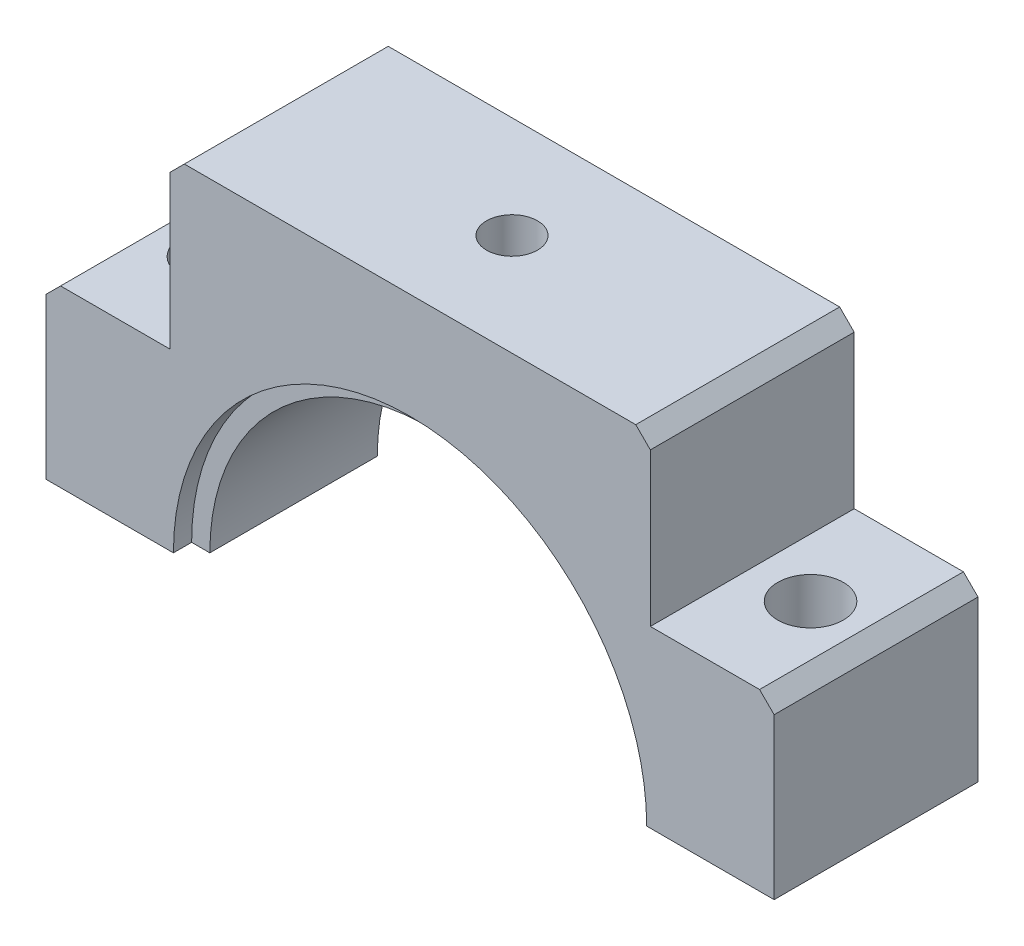
from build123d import *

# Parameters (mm, degrees)
BOSS_EXTRUDE1_DEPTH       = 28
CHAMFER1_SIZE             = 2
M8X1_0_TAPPED_HOLE1_D     = 7
M8X1_0_TAPPED_HOLE1_DEPTH = 13
M8X1_0_TAPPED_HOLE1_TIP   = 2.103012167
HOLE2_D                   = 9
SKETCH15_R                = 32.5
CUT_EXTRUDE3_DEPTH        = 2.5
CUT_EXTRUDE4_START        = -2.5
SKETCH16_R                = 32.5
CUT_EXTRUDE4_DEPTH        = 2.5
HOLE3_D                   = 4


with BuildPart() as part:
    # Sketch1 → Boss-Extrude1 (new body)
    with BuildSketch(Plane.XY):
        with BuildLine():
            Line((-50, 24), (-33, 24))
            Line((-33, 24), (-33, 47))
            Line((-33, 47), (33, 47))
            Line((33, 47), (33, 24))
            Line((33, 24), (50, 24))
            Line((50, 24), (50, 0))
            Line((50, 0), (30, 0))
            ThreePointArc((30, 0), (0, 30), (-30, 0))
            Line((-30, 0), (-50, 0))
            Line((-50, 0), (-50, 24))
        make_face()
    extrude(amount=BOSS_EXTRUDE1_DEPTH)

    # Chamfer1
    chamfer1_edges = [part.edges().sort_by_distance(p)[0] for p in [
        (-50, 24, 14),
        (-33, 47, 14),
        (33, 47, 14),
        (50, 24, 14),
    ]]
    chamfer(chamfer1_edges, length=CHAMFER1_SIZE)

    # M8x1.0 Tapped Hole1
    with Locations(Plane(origin=(0, 47, 0), x_dir=(1, 0, 0), z_dir=(0, 1, 0))):
        with Locations((0, -14)):
            Hole(M8X1_0_TAPPED_HOLE1_D / 2, depth=M8X1_0_TAPPED_HOLE1_DEPTH)
            with Locations((0, 0, -(M8X1_0_TAPPED_HOLE1_DEPTH + M8X1_0_TAPPED_HOLE1_TIP / 2))):  # 118° drill point
                Cone(0, M8X1_0_TAPPED_HOLE1_D / 2, M8X1_0_TAPPED_HOLE1_TIP, mode=Mode.SUBTRACT)

    # Hole2 (through all)
    with Locations(Plane(origin=(0, 24, 0), x_dir=(1, 0, 0), z_dir=(0, 1, 0))):
        with Locations((-41, -14), (41, -14)):
            Hole(HOLE2_D / 2)

    # Sketch15 → Cut-Extrude3 (cut)
    with BuildSketch(Plane(origin=(0, 0, 0), x_dir=(-1, 0, 0), z_dir=(0, 0, -1))):
        Circle(SKETCH15_R)
    extrude(amount=-CUT_EXTRUDE3_DEPTH, mode=Mode.SUBTRACT)

    # Sketch16 → Cut-Extrude4 (cut)
    with BuildSketch(Plane.XY.offset(28).offset(CUT_EXTRUDE4_START)):
        Circle(SKETCH16_R)
    extrude(amount=CUT_EXTRUDE4_DEPTH, mode=Mode.SUBTRACT)

    # Hole3 (through all)
    with Locations(Plane(origin=(0, 47, 0), x_dir=(1, 0, 0), z_dir=(0, 1, 0))):
        with Locations((0, -14)):
            Hole(HOLE3_D / 2)


solid = part.part
